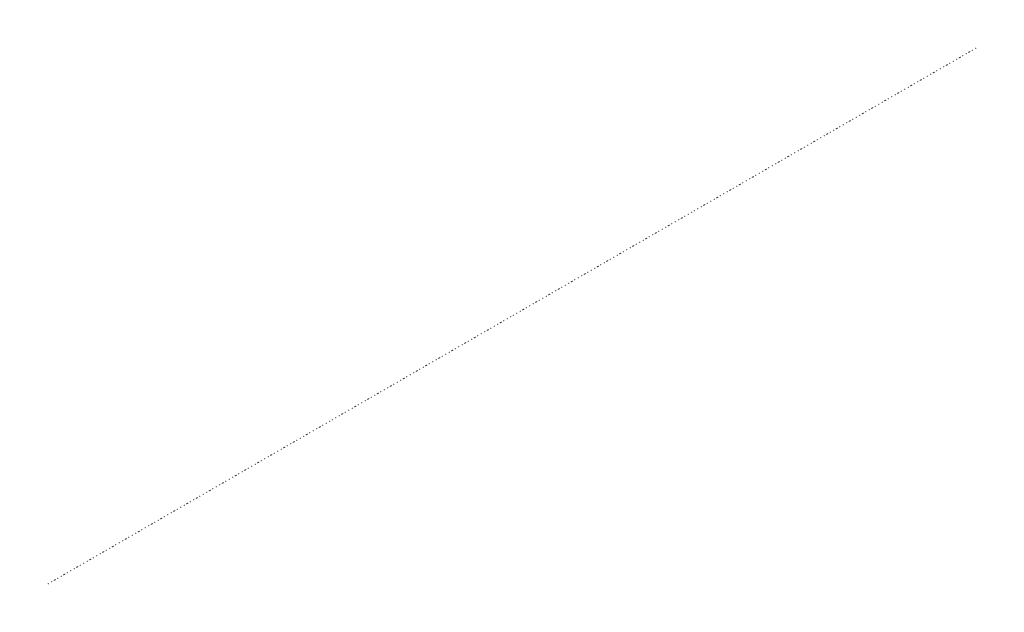
SolidWorks part; units mm, degrees
ref_plane "Front Plane" through (0, 0, 0) normal (0, 0, 1) x (1, 0, 0)
ref_plane "Top Plane" through (0, 0, 0) normal (0, 1, 0) x (1, 0, 0)
ref_plane "Right Plane" through (0, 0, 0) normal (1, 0, 0) x (0, 0, -1)
sketch "Sketch1" plane through (0, 0, 0) normal (0, 0, 1) x (1, 0, 0)
  circle A0 centre (0, 0) radius 0.0625
  dimension "D1" = 0.125
extrude "Boss-Extrude1" add sketch "Sketch1" along normal blind 1900
